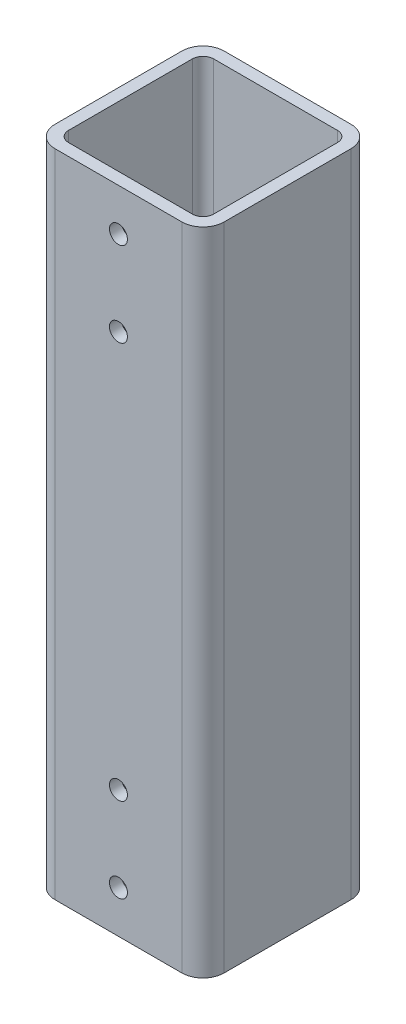
from build123d import *

# Parameters (mm, degrees)
SKETCH1_W                      = 307.64
SKETCH1_H                      = 80
BOSS_EXTRUDE1_DEPTH            = 80
SKETCH2_W                      = 68.6
SKETCH2_H                      = 68.6
CUT_EXTRUDE1_DEPTH             = 314.476266406
F_8_5_8_5_DIAMETER_HOLE2_D     = 8.5
F_8_5_8_5_DIAMETER_HOLE2_DEPTH = 5.7
FILLET1_R                      = 5
FILLET2_R                      = 10
F_8_5_8_5_DIAMETER_HOLE3_D     = 8.5
F_8_5_8_5_DIAMETER_HOLE3_DEPTH = 10
F_8_5_8_5_DIAMETER_HOLE3_TIP   = 2.553657631
F_8_5_8_5_DIAMETER_HOLE5_D     = 8.5
F_8_5_8_5_DIAMETER_HOLE5_DEPTH = 10
F_8_5_8_5_DIAMETER_HOLE5_TIP   = 2.553657631


with BuildPart() as part:
    # Sketch1 → Boss-Extrude1 (new body)
    with BuildSketch(Plane(origin=(-35, 0, 0), x_dir=(0, -1, 0), z_dir=(-1, 0, 0))):
        with Locations((95.322857143, 0)):
            Rectangle(SKETCH1_W, SKETCH1_H)
    extrude(amount=-BOSS_EXTRUDE1_DEPTH)

    # Sketch2 → Cut-Extrude1 (cut, through all)
    with BuildSketch(Plane.XZ.offset(249.142857143)):
        with Locations((5, 0)):
            Rectangle(SKETCH2_W, SKETCH2_H)
    extrude(amount=-CUT_EXTRUDE1_DEPTH, mode=Mode.SUBTRACT)

    # Ø8.5 (8.5) Diameter Hole2
    with Locations(Plane.XY.offset(40)):
        with Locations((5, -189.142857143), (5, -229.142857143)):
            Hole(F_8_5_8_5_DIAMETER_HOLE2_D / 2, depth=F_8_5_8_5_DIAMETER_HOLE2_DEPTH)

    # Fillet1
    fillet1_edges = [part.edges().sort_by_distance(p)[0] for p in [
        (-29.3, -95.322857143, -34.3),
        (-29.3, -95.322857143, 34.3),
        (39.3, -95.322857143, 34.3),
        (39.3, -95.322857143, -34.3),
    ]]
    fillet(fillet1_edges, radius=FILLET1_R)

    # Fillet2
    fillet2_edges = [part.edges().sort_by_distance(p)[0] for p in [
        (45, -95.322857143, 40),
        (45, -95.322857143, -40),
        (-35, -95.322857143, 40),
        (-35, -95.322857143, -40),
    ]]
    fillet(fillet2_edges, radius=FILLET2_R)

    # Ø8.5 (8.5) Diameter Hole3
    with Locations(Plane.XY.offset(40)):
        with Locations((5, 38.497142857)):
            Hole(F_8_5_8_5_DIAMETER_HOLE3_D / 2, depth=F_8_5_8_5_DIAMETER_HOLE3_DEPTH)
            with Locations((0, 0, -(F_8_5_8_5_DIAMETER_HOLE3_DEPTH + F_8_5_8_5_DIAMETER_HOLE3_TIP / 2))):  # 118° drill point
                Cone(0, F_8_5_8_5_DIAMETER_HOLE3_D / 2, F_8_5_8_5_DIAMETER_HOLE3_TIP, mode=Mode.SUBTRACT)

    # Ø8.5 (8.5) Diameter Hole5
    with Locations(Plane.XY.offset(40)):
        with Locations((5, -1.502857143)):
            Hole(F_8_5_8_5_DIAMETER_HOLE5_D / 2, depth=F_8_5_8_5_DIAMETER_HOLE5_DEPTH)
            with Locations((0, 0, -(F_8_5_8_5_DIAMETER_HOLE5_DEPTH + F_8_5_8_5_DIAMETER_HOLE5_TIP / 2))):  # 118° drill point
                Cone(0, F_8_5_8_5_DIAMETER_HOLE5_D / 2, F_8_5_8_5_DIAMETER_HOLE5_TIP, mode=Mode.SUBTRACT)


solid = part.part
